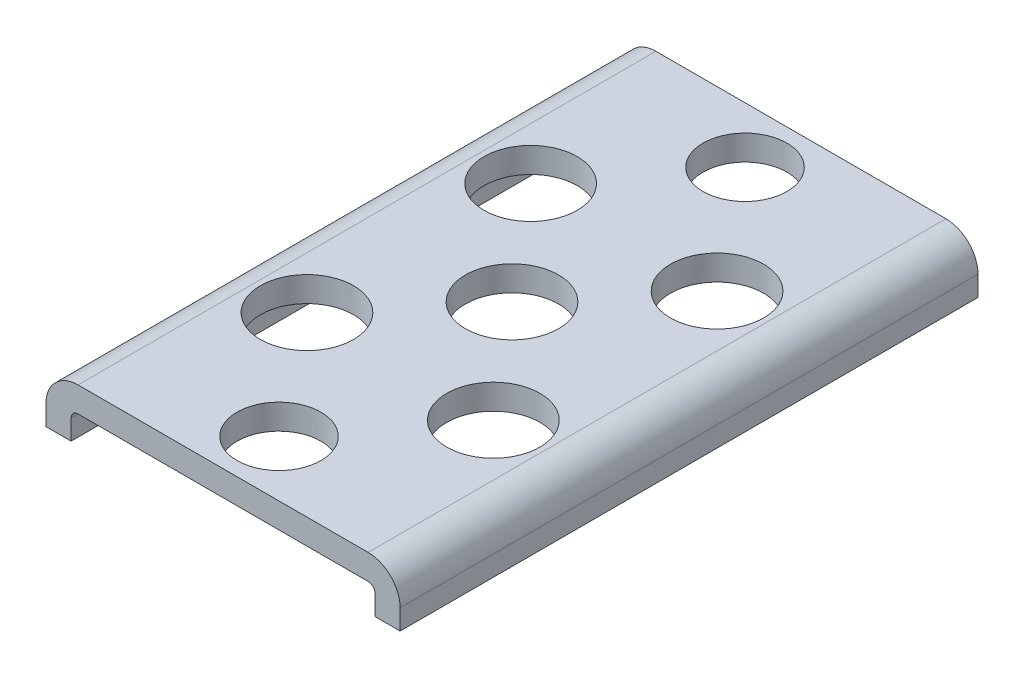
from build123d import *

# Parameters (mm, degrees)
SKETCH1_W                      = 37.995749454
SKETCH1_H                      = 62
BOSS_EXTRUDE1_DEPTH            = 5.594860996
SKETCH2_W                      = 32.595749454
SKETCH2_H                      = 2.894860996
CUT_EXTRUDE1_DEPTH             = 66.086263633
F_10_0_10_DIAMETER_HOLE1_D     = 10
F_10_0_10_DIAMETER_HOLE1_DEPTH = 5.594860996
F_9_0_9_DIAMETER_HOLE1_D       = 9
F_9_0_9_DIAMETER_HOLE1_DEPTH   = 5.594860996
FILLET1_R                      = 0.7366
FILLET2_R                      = 3.4366


with BuildPart() as part:
    # Sketch1 → Boss-Extrude1 (new body)
    with BuildSketch(Plane(origin=(0, 0, 0), x_dir=(1, 0, 0), z_dir=(0, 1, 0))):
        with Locations((0, 45)):
            Rectangle(SKETCH1_W, SKETCH1_H)
    extrude(amount=-BOSS_EXTRUDE1_DEPTH)

    # Sketch2 → Cut-Extrude1 (cut, through all)
    with BuildSketch(Plane(origin=(0, 0, -76), x_dir=(-1, 0, 0), z_dir=(0, 0, -1))):
        with Locations((0, -4.147430498)):
            Rectangle(SKETCH2_W, SKETCH2_H)
    extrude(amount=-CUT_EXTRUDE1_DEPTH, mode=Mode.SUBTRACT)

    # Ø10.0 (10) Diameter Hole1
    with Locations(Plane(origin=(0, 0, 0), x_dir=(1, 0, 0), z_dir=(0, 1, 0))):
        with Locations((0, 45), (-10, 57), (-10, 33), (10, 33), (10, 57)):
            Hole(F_10_0_10_DIAMETER_HOLE1_D / 2, depth=F_10_0_10_DIAMETER_HOLE1_DEPTH)

    # Ø9.0 (9) Diameter Hole1
    with Locations(Plane(origin=(0, 0, 0), x_dir=(1, 0, 0), z_dir=(0, 1, 0))):
        with Locations((0, 70), (0, 20)):
            Hole(F_9_0_9_DIAMETER_HOLE1_D / 2, depth=F_9_0_9_DIAMETER_HOLE1_DEPTH)

    # Fillet1
    fillet1_edges = [part.edges().sort_by_distance(p)[0] for p in [
        (16.297874727, -2.7, -45),
        (-16.297874727, -2.7, -45),
    ]]
    fillet(fillet1_edges, radius=FILLET1_R)

    # Fillet2
    fillet2_edges = [part.edges().sort_by_distance(p)[0] for p in [
        (18.997874727, 0, -45),
        (-18.997874727, 0, -45),
    ]]
    fillet(fillet2_edges, radius=FILLET2_R)


solid = part.part
